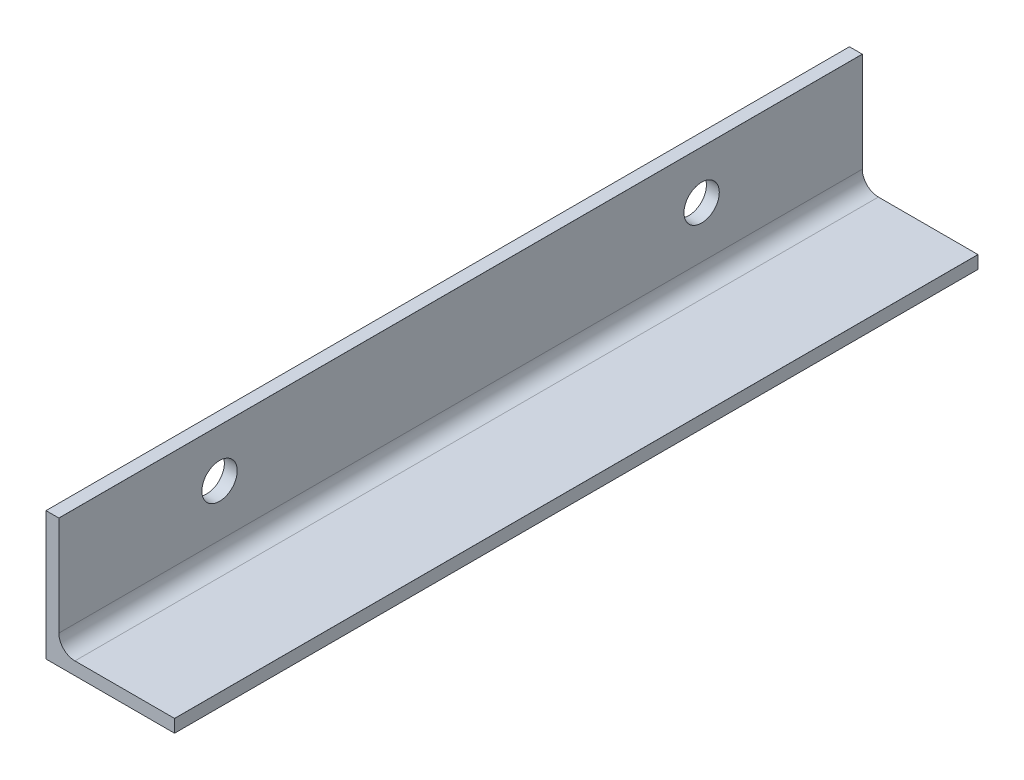
SolidWorks part; units mm, degrees
material "热轧等边角钢 Q235A"
ref_plane "前视基准面" through (0, 0, 0) normal (0, 0, 1) x (1, 0, 0)
ref_plane "上视基准面" through (0, 0, 0) normal (0, 1, 0) x (1, 0, 0)
ref_plane "右视基准面" through (0, 0, 0) normal (1, 0, 0) x (0, 0, -1)
sketch "草图1" plane through (0, 0, 0) normal (0, 0, 1) x (1, 0, 0)
  line L0 (0, 0) -> (0, 40)
  line L1 (0, 40) -> (3.99, 40)
  line L2 (4, 39.99) -> (4, 9)
  line L3 (9, 4) -> (39.99, 4)
  line L4 (40, 3.99) -> (40, 0)
  line L5 (40, 0) -> (0, 0)
  arc A0 (4, 39.99) -> (3.99, 40) centre (3.99, 39.99) ccw
  arc A1 (9, 4) -> (4, 9) centre (9, 9) cw
  arc A2 (40, 3.99) -> (39.99, 4) centre (39.99, 3.99) ccw
  point P9 (4, 40)
  point P14 (40, 4)
extrude "拉伸1" add sketch "草图1" along normal blind 250
hole_wizard "Ø11.0 (11) 直径孔1" positions "草图5" profile "草图4" hole size "Ø11.0" standard "Gb"
sketch "草图5" plane through (0, 0, 0) normal (-1, 0, 0) x (0, 0, 1)
  line L0 (250, 40) -> (0, 40) construction
  line L3 (250, 40) -> (250, 0) construction
  line L4 (0, 40) -> (0, 0) construction
  point P0 (200, 25)
  point P2 (50, 25)
  dimension "D1" = 15
  dimension "D2" = 50
  dimension "D3" = 50
  dimension "D4" = 15
sketch "草图4" plane through (0, 25, 200) normal (0, 1, 0) x (0, 0, 1)
  line L0 (0, 0) -> (0, 13.3047)
  line L1 (0, 13.3047) -> (5.5, 10)
  line L2 (5.5, 10) -> (5.5, 0)
  line L5 (5.5, 0) -> (0, 0)
  line L10 (0, 13.3047) -> (-5.5, 10) construction
  line L11 (0, -6.35) -> (0, 107.95) construction
  dimension "孔直径" = 11
  dimension "孔深度" = 10
  dimension "导头角度" = 118
equation "\"D2@草图1\" = \"D1@草图1\""
equation "\"D4@草图1\" = \"D3@草图1\""
equation "\"D7@草图1\" = \"D5@草图1\""
